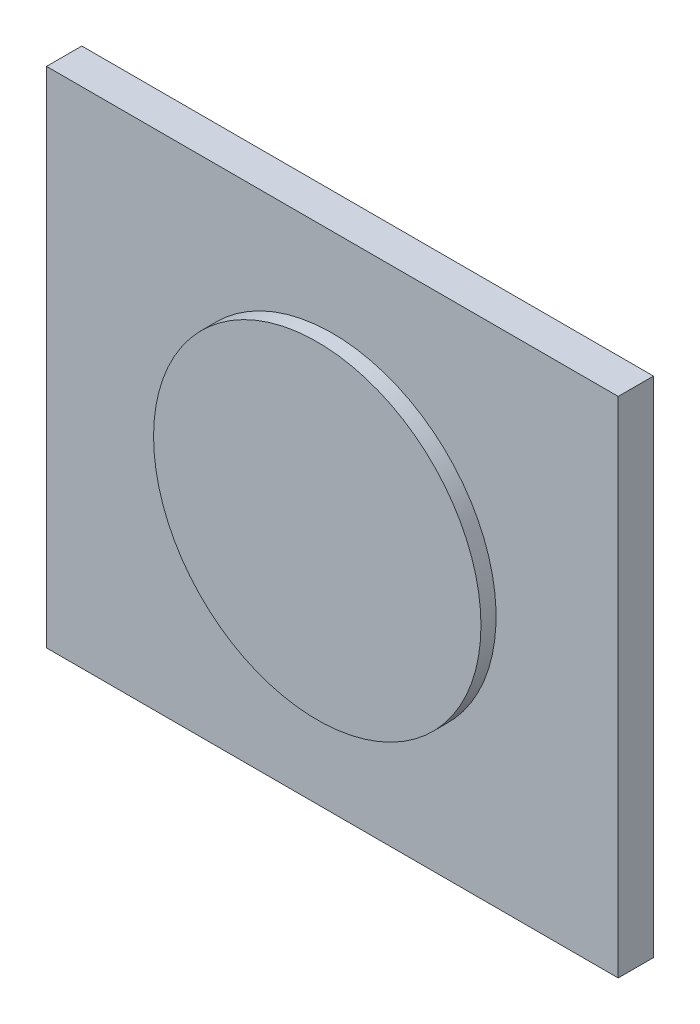
SolidWorks part; units mm, degrees
material "普通碳钢"
ref_plane "Front Plane" through (0, 0, 0) normal (0, 0, 1) x (1, 0, 0)
ref_plane "Top Plane" through (0, 0, 0) normal (0, 1, 0) x (1, 0, 0)
ref_plane "Right Plane" through (0, 0, 0) normal (1, 0, 0) x (0, 0, -1)
sketch "Sketch1" plane through (0, 0, 0) normal (0, 0, 1) x (1, 0, 0)
  line L0 (0, 0) -> (0, 200)
  line L1 (0, 200) -> (227, 200)
  line L2 (227, 200) -> (227, 0)
  line L3 (227, 0) -> (0, 0)
  dimension "D1" = 227
  dimension "D2" = 200
extrude "Boss-Extrude1" add sketch "Sketch1" along normal blind 14
sketch "Sketch2" plane through (0, 0, 14) normal (0, 0, 1) x (1, 0, 0)
  line L0 (0, 100) -> (227, 100) construction
  line L1 (0, 200) -> (0, 0) construction
  line L2 (227, 0) -> (227, 200) construction
  circle A0 centre (113.5, 100) radius 65
  dimension "D1" = 130
extrude "Boss-Extrude2" add sketch "Sketch2" along normal blind 6
sketch "Sketch3" plane through (0, 0, 0) normal (0, 0, -1) x (-1, 0, 0)
  circle A0 centre (-113.5, 100) radius 65 construction
  circle A1 centre (-113.5, 100) radius 65 construction
  circle A2 centre (-113.5, 100) radius 70
  dimension "D1" = 140
extrude "Boss-Extrude3" add sketch "Sketch3" along normal blind 8
